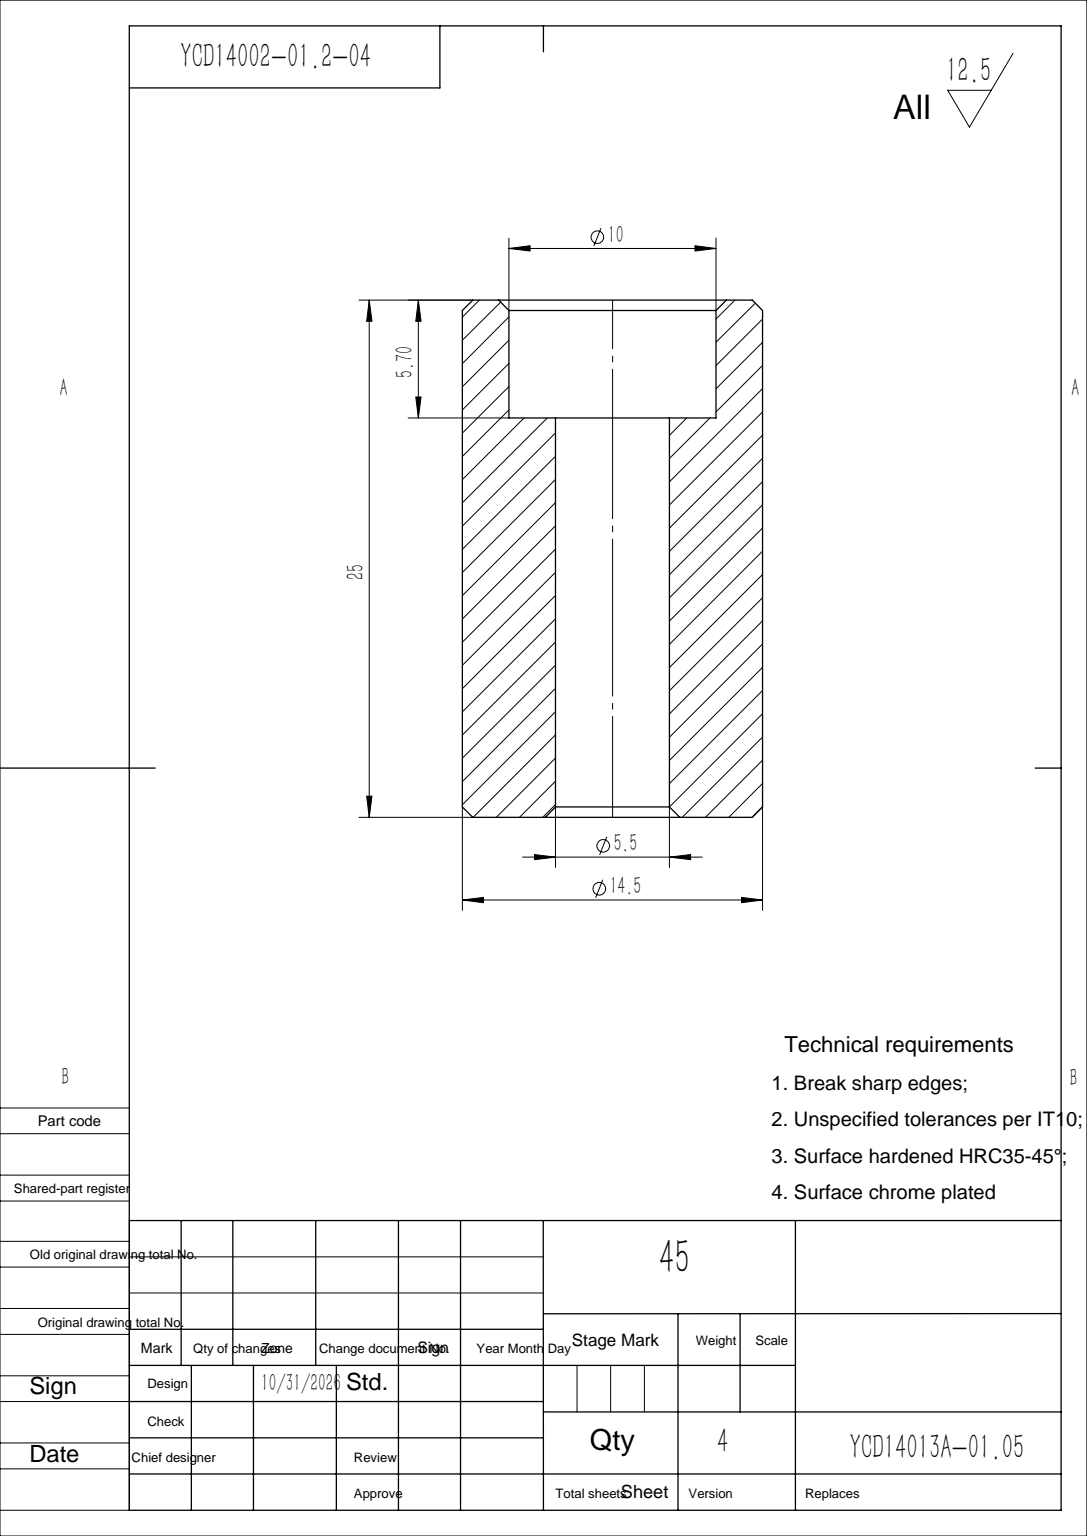
SolidWorks part; units mm, degrees
material "45"
ref_plane "Front Plane" through (0, 0, 0) normal (0, 0, 1) x (1, 0, 0)
ref_plane "Top Plane" through (0, 0, 0) normal (0, 1, 0) x (1, 0, 0)
ref_plane "Right Plane" through (0, 0, 0) normal (1, 0, 0) x (0, 0, -1)
sketch "Sketch1" plane through (0, 0, 0) normal (0, 1, 0) x (1, 0, 0)
  circle A0 centre (0, 0) radius 7.25
  dimension "D1" = 14.5
extrude "Boss-Extrude1" add sketch "Sketch1" along normal blind 25
hole_wizard "Hole Size by Hex Socket Screw Type1" positions "Sketch5" profile "Sketch4" counterbore size "M5" standard "Gb" end condition through all
sketch "Sketch5" plane through (0, 25, 0) normal (0, 1, 0) x (1, 0, 0)
  point P0 (0, 0)
sketch "Sketch4" plane through (0, 25, 0) normal (1, 0, 0) x (0, 0, 1)
  line L0 (0, 0) -> (0, 25)
  line L1 (0, 25) -> (2.75, 25)
  line L3 (2.75, 25) -> (2.75, 5.7)
  line L4 (2.75, 5.7) -> (5, 5.7)
  line L5 (5, 5.7) -> (5, 0)
  line L7 (5, 0) -> (0, 0)
  line L11 (0, -6.35) -> (0, 107.95) construction
  dimension "通孔孔直径" = 5.5
  dimension "通孔孔深度" = 25
  dimension "柱形沉头孔直径" = 10
  dimension "柱形沉头孔深度" = 5.7
chamfer "Chamfer1" distance 0.5 angle 45 4 edges at (0, 25, 7.25) (0, 25, 5) (0, 0, 7.25) (0, 0, 2.75)
